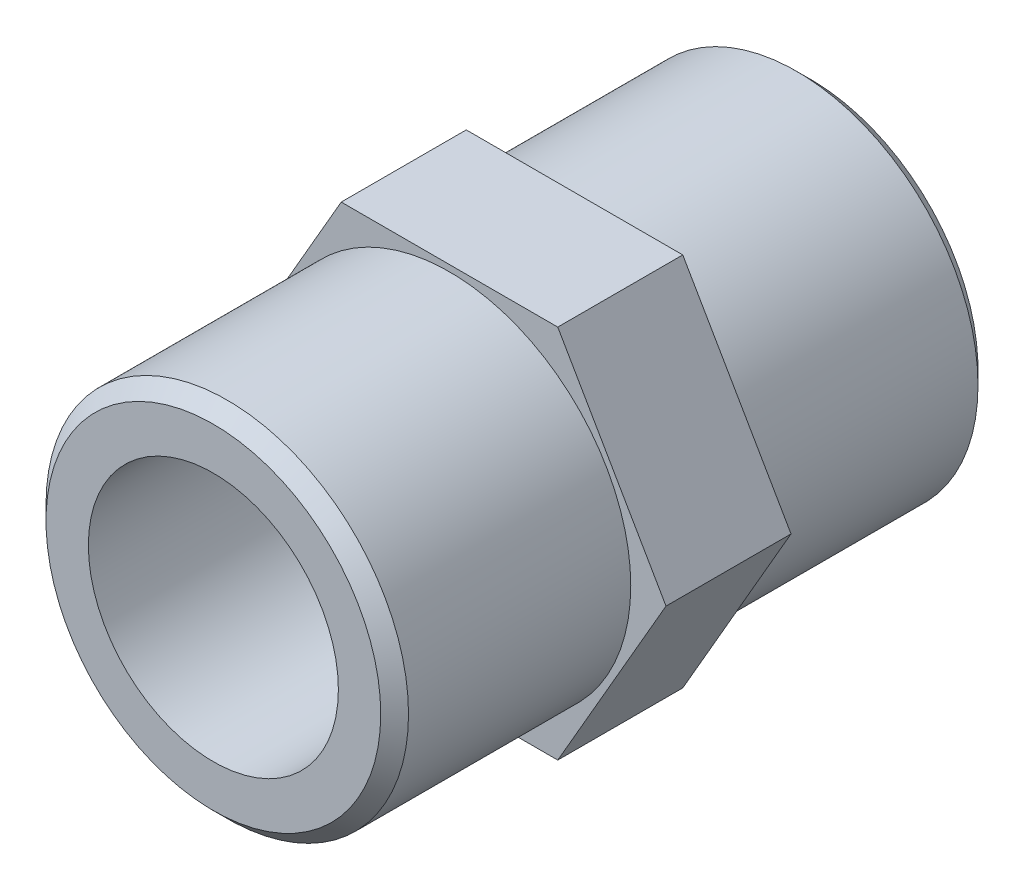
from build123d import *

# Parameters (mm, degrees)
EXTRUDE_1_DEPTH     = 4.5
SKETCH_4_R          = 13.05
EXTRUDE_3_DEPTH     = 17
CUT_EXTRUDE_2_REACH = 49.689
SKETCH_5_R          = 9
CHAMFER_1_SIZE      = 1


with BuildPart() as part:
    # 草图1 → 凸台-拉伸1 (new, symmetric)
    with BuildSketch(Plane.XY):
        Polygon((15.588457268, 0), (7.794228634, 13.5), (-7.794228634, 13.5), (-15.588457268, 0), (-7.794228634, -13.5), (7.794228634, -13.5), align=None)
    extrude(amount=EXTRUDE_1_DEPTH, both=True)

    # 草图4 → 凸台-拉伸3 (add)
    with BuildSketch(Plane(origin=(0, 0, -4.5), x_dir=(-1, 0, 0), z_dir=(0, 0, -1))):
        Circle(SKETCH_4_R)
    extrude_3 = extrude(amount=EXTRUDE_3_DEPTH)

    # 镜向1: 凸台-拉伸3 across plane
    add(extrude_3.mirror(Plane.XY))

    # 草图5 → 切除-拉伸2 (cut, up to next)
    with BuildSketch(Plane(origin=(0, 0, -21.5), x_dir=(-1, 0, 0), z_dir=(0, 0, -1)), mode=Mode.PRIVATE) as cut_extrude_2_sk1:
        Circle(SKETCH_5_R)
    cut_extrude_2_tool1 = extrude(cut_extrude_2_sk1.sketch, amount=-CUT_EXTRUDE_2_REACH, mode=Mode.PRIVATE) & part.part
    add(cut_extrude_2_tool1.solids().sort_by_distance((0, 0, -21.5))[0], mode=Mode.SUBTRACT)

    # 倒角1
    chamfer_1_edges = [part.edges().sort_by_distance(p)[0] for p in [
        (13.05, 0, -21.5),
        (13.05, 0, 21.5),
    ]]
    chamfer(chamfer_1_edges, length=CHAMFER_1_SIZE)


solid = part.part
